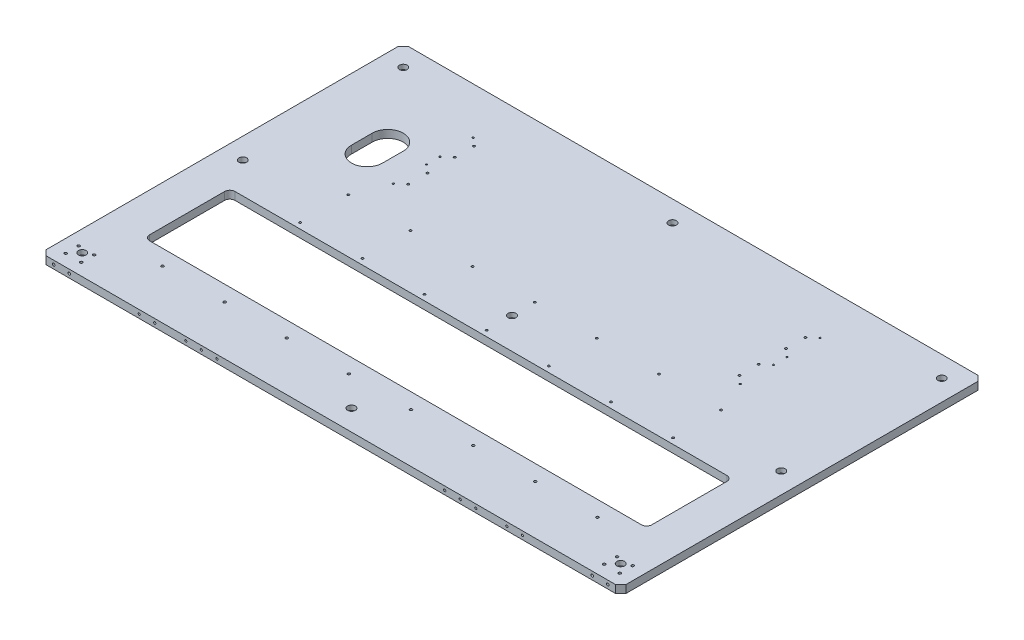
SolidWorks part; units mm, degrees
material "S45C"
ref_plane "前视基准面" through (0, 0, 0) normal (0, 0, 1) x (1, 0, 0)
ref_plane "上视基准面" through (0, 0, 0) normal (0, 1, 0) x (1, 0, 0)
ref_plane "右视基准面" through (0, 0, 0) normal (1, 0, 0) x (0, 0, -1)
sketch "草图1" plane through (0, 0, 0) normal (0, 1, 0) x (1, 0, 0)
  line L1 (-560, 350) -> (560, 350)
  line L2 (-560, 350) -> (-560, -350)
  line L3 (-560, -350) -> (560, -350)
  line L4 (560, 350) -> (560, -350)
  line L5 (-560, 350) -> (560, -350) construction
  line L6 (-560, -350) -> (560, 350) construction
  point P0 (0, 0)
  dimension "D1" = 1120
  dimension "D2" = 700
extrude "凸台-拉伸1" add sketch "草图1" along normal blind 15
chamfer "倒角1" distance 10 angle 45 4 edges at (-560, 7.5, -350) (560, 7.5, -350) (560, 7.5, 350) (-560, 7.5, 350)
sketch "草图2" plane through (0, 15, 0) normal (0, 1, 0) x (1, 0, 0)
  line L0 (560, -340) -> (560, 340) construction
  line L1 (485, -60) -> (-485, -60)
  line L2 (485, -60) -> (485, -225)
  line L3 (485, -225) -> (-485, -225)
  line L4 (-485, -60) -> (-485, -225)
  line L5 (-560, 340) -> (-560, -340) construction
  line L6 (-550, -350) -> (550, -350) construction
  dimension "D1" = 75
  dimension "D2" = 75
  dimension "D3" = 125
  dimension "D4" = 165
extrude "切除-拉伸1" cut sketch "草图2" against normal blind 20
fillet "圆角1" radius 10 4 edges at (485, 7.5, 60) (485, 7.5, 225) (-485, 7.5, 225) (-485, 7.5, 60)
hole_wizard "打孔尺寸(%根据)内六角圆柱头螺钉的类型1" positions "草图3" profile "草图4" counterbore size "M8" standard "GB"
sketch "草图3" plane through (0, 15, 0) normal (0, 1, 0) x (1, 0, 0)
  point P0 (520, -310)
  point P3 (520, 0)
  point P6 (520, 310)
  point P9 (-520, -310)
  point P12 (-520, 0)
  point P15 (-520, 310)
sketch "草图4" plane through (520, 15, 310) normal (1, 0, 0) x (0, 0, 1)
  line L0 (0, 0) -> (0, 22.4539)
  line L1 (0, 22.4539) -> (4.5, 19.75)
  line L2 (4.5, 19.75) -> (4.5, 9)
  line L3 (4.5, 9) -> (7.5, 9)
  line L4 (7.5, 9) -> (7.5, 0)
  line L5 (7.5, 0) -> (0, 0)
  line L10 (0, 22.4539) -> (-4.5, 19.75) construction
  line L11 (0, -6.35) -> (0, 107.95) construction
  dimension "孔直径" = 9
  dimension "孔深度" = 19.75
  dimension "柱形沉头孔直径" = 15
  dimension "柱形沉头孔深度" = 9
  dimension "导头角度" = 118
hole_wizard "M6 螺纹孔1" positions "草图5" profile "草图6" tap size "M6" standard "GB"
sketch "草图5" plane through (0, 15, 0) normal (0, 1, 0) x (1, 0, 0)
  point P0 (-420, -255)
  point P3 (-300, -255)
  point P6 (-180, -255)
  point P9 (-60, -255)
  point P12 (60, -255)
  point P15 (180, -255)
  point P18 (300, -255)
  point P21 (420, -255)
sketch "草图6" plane through (-420, 15, 255) normal (1, 0, 0) x (0, 0, 1)
  line L0 (0, 0) -> (0, 16.5022)
  line L1 (0, 16.5022) -> (2.5, 15)
  line L2 (2.5, 15) -> (2.5, 0)
  line L5 (2.5, 0) -> (0, 0)
  line L10 (0, 16.5022) -> (-2.5, 15) construction
  line L11 (0, -6.35) -> (0, 107.95) construction
  dimension "螺纹孔钻头直径" = 5
  dimension "螺纹孔钻头深度" = 15
  dimension "导头角度" = 118
cosmetic thread "孔螺蚊线31" parameters "D1"=12, "D2"=6
cosmetic thread "孔螺蚊线32" parameters "D1"=12, "D2"=6
cosmetic thread "孔螺蚊线33" parameters "D1"=12, "D2"=6
cosmetic thread "孔螺蚊线34" parameters "D1"=12, "D2"=6
cosmetic thread "孔螺蚊线35" parameters "D1"=12, "D2"=6
cosmetic thread "孔螺蚊线36" parameters "D1"=12, "D2"=6
cosmetic thread "孔螺蚊线37" parameters "D1"=12, "D2"=6
cosmetic thread "孔螺蚊线38" parameters "D1"=12, "D2"=6
hole_wizard "M5 螺纹孔1" positions "草图7" profile "草图8" tap size "M5" standard "GB"
sketch "草图7" plane through (0, 15, 0) normal (0, 1, 0) x (1, 0, 0)
  point P0 (360, -49)
  point P3 (360, 44)
  point P6 (240, -49)
  point P9 (240, 44)
  point P12 (120, -49)
  point P15 (120, 44)
  point P18 (0, -49)
  point P21 (0, 44)
  point P24 (-120, -49)
  point P27 (-120, 44)
  point P30 (-240, -49)
  point P33 (-240, 44)
  point P36 (-360, -49)
  point P39 (-360, 44)
sketch "草图8" plane through (360, 15, 49) normal (1, 0, 0) x (0, 0, 1)
  line L0 (0, 0) -> (0, 21.2618)
  line L1 (0, 21.2618) -> (2.1, 20)
  line L2 (2.1, 20) -> (2.1, 0)
  line L5 (2.1, 0) -> (0, 0)
  line L10 (0, 21.2618) -> (-2.1, 20) construction
  line L11 (0, -6.35) -> (0, 107.95) construction
  dimension "螺纹孔钻头直径" = 4.2
  dimension "螺纹孔钻头深度" = 20
  dimension "导头角度" = 118
cosmetic thread "孔螺蚊线9" parameters "D1"=10, "D2"=5
cosmetic thread "孔螺蚊线10" parameters "D1"=10, "D2"=5
cosmetic thread "孔螺蚊线11" parameters "D1"=10, "D2"=5
cosmetic thread "孔螺蚊线12" parameters "D1"=10, "D2"=5
cosmetic thread "孔螺蚊线13" parameters "D1"=10, "D2"=5
cosmetic thread "孔螺蚊线14" parameters "D1"=10, "D2"=5
cosmetic thread "孔螺蚊线15" parameters "D1"=10, "D2"=5
cosmetic thread "孔螺蚊线16" parameters "D1"=10, "D2"=5
cosmetic thread "孔螺蚊线17" parameters "D1"=10, "D2"=5
cosmetic thread "孔螺蚊线18" parameters "D1"=10, "D2"=5
cosmetic thread "孔螺蚊线19" parameters "D1"=10, "D2"=5
cosmetic thread "孔螺蚊线20" parameters "D1"=10, "D2"=5
cosmetic thread "孔螺蚊线21" parameters "D1"=10, "D2"=5
cosmetic thread "孔螺蚊线22" parameters "D1"=10, "D2"=5
sketch "草图9" plane through (0, 15, 0) normal (0, 1, 0) x (1, 0, 0)
  line L0 (-410, 130) -> (-410, 170) construction
  line L1 (-440, 130) -> (-440, 170)
  line L2 (-380, 130) -> (-380, 170)
  line L3 (550, 350) -> (-550, 350) construction
  line L4 (-560, 340) -> (-560, -340) construction
  arc A0 (-440, 130) -> (-380, 130) centre (-410, 130) ccw
  arc A1 (-380, 170) -> (-440, 170) centre (-410, 170) ccw
  point P2 (-410, 150)
  dimension "D1" = 180
  dimension "D3" = 150
  dimension "D4" = 30
  dimension "D2" = 40
extrude "切除-拉伸2" cut sketch "草图9" against normal blind 20
hole_wizard "M5 螺纹孔2" positions "草图10" profile "草图11" tap size "M5" standard "GB"
sketch "草图10" plane through (0, 0, 350) normal (0, 0, 1) x (1, 0, 0)
  line L1 (-550, 15) -> (550, 15) construction
  line L2 (560, 15) -> (560, 0) construction
  point P0 (-280, 7.5)
  point P3 (-250, 7.5)
  point P6 (-220, 7.5)
  point P10 (280, 7.5)
  point P12 (250, 7.5)
  point P14 (220, 7.5)
  dimension "D1" = 30
  dimension "D2" = 30
  dimension "D3" = 7.5
  dimension "D4" = 280
sketch "草图11" plane through (-280, 7.5, 350) normal (1, 0, 0) x (0, -1, 0)
  line L0 (0, 0) -> (0, 21.2618)
  line L1 (0, 21.2618) -> (2.1, 20)
  line L2 (2.1, 20) -> (2.1, 0)
  line L5 (2.1, 0) -> (0, 0)
  line L10 (0, 21.2618) -> (-2.1, 20) construction
  line L11 (0, -6.35) -> (0, 107.95) construction
  dimension "螺纹孔钻头直径" = 4.2
  dimension "螺纹孔钻头深度" = 20
  dimension "导头角度" = 118
cosmetic thread "孔螺蚊线39" parameters "D1"=10, "D2"=5
cosmetic thread "孔螺蚊线40" parameters "D1"=10, "D2"=5
cosmetic thread "孔螺蚊线41" parameters "D1"=10, "D2"=5
cosmetic thread "孔螺蚊线58" parameters "D1"=10, "D2"=5
cosmetic thread "孔螺蚊线59" parameters "D1"=10, "D2"=5
cosmetic thread "孔螺蚊线60" parameters "D1"=10, "D2"=5
hole_wizard "M4 螺纹孔1" positions "草图12" profile "草图13" tap size "M4" standard "GB"
sketch "草图12" plane through (0, 15, 0) normal (0, 1, 0) x (1, 0, 0)
  point P0 (335, 106)
  point P3 (335, 170)
  point P6 (-335, 106)
  point P9 (-335, 170)
  point P12 (-335, 196)
  point P15 (-335, 260)
  point P18 (335, 196)
  point P21 (335, 260)
sketch "草图13" plane through (335, 15, -106) normal (1, 0, 0) x (0, 0, 1)
  line L0 (0, 0) -> (0, 20.9914)
  line L1 (0, 20.9914) -> (1.65, 20)
  line L2 (1.65, 20) -> (1.65, 0)
  line L5 (1.65, 0) -> (0, 0)
  line L10 (0, 20.9914) -> (-1.65, 20) construction
  line L11 (0, -6.35) -> (0, 107.95) construction
  dimension "螺纹孔钻头直径" = 3.3
  dimension "螺纹孔钻头深度" = 20
  dimension "导头角度" = 118
cosmetic thread "孔螺蚊线42" parameters "D1"=8, "D2"=4
cosmetic thread "孔螺蚊线43" parameters "D1"=8, "D2"=4
cosmetic thread "孔螺蚊线44" parameters "D1"=8, "D2"=4
cosmetic thread "孔螺蚊线45" parameters "D1"=8, "D2"=4
cosmetic thread "孔螺蚊线46" parameters "D1"=8, "D2"=4
cosmetic thread "孔螺蚊线47" parameters "D1"=8, "D2"=4
cosmetic thread "孔螺蚊线48" parameters "D1"=8, "D2"=4
cosmetic thread "孔螺蚊线49" parameters "D1"=8, "D2"=4
hole_wizard "M5 螺纹孔3" positions "草图14" profile "草图15" tap size "M5" standard "GB"
sketch "草图14" plane through (0, 15, 0) normal (0, 1, 0) x (1, 0, 0)
  point P0 (320, 119.5)
  point P3 (320, 156.5)
  point P6 (320, 209.5)
  point P9 (320, 246.5)
  point P12 (-320, 119.5)
  point P15 (-320, 156.5)
  point P18 (-320, 209.5)
  point P21 (-320, 246.5)
sketch "草图15" plane through (320, 15, -119.5) normal (1, 0, 0) x (0, 0, 1)
  line L0 (0, 0) -> (0, 21.2618)
  line L1 (0, 21.2618) -> (2.1, 20)
  line L2 (2.1, 20) -> (2.1, 0)
  line L5 (2.1, 0) -> (0, 0)
  line L10 (0, 21.2618) -> (-2.1, 20) construction
  line L11 (0, -6.35) -> (0, 107.95) construction
  dimension "螺纹孔钻头直径" = 4.2
  dimension "螺纹孔钻头深度" = 20
  dimension "导头角度" = 118
cosmetic thread "孔螺蚊线50" parameters "D1"=10, "D2"=5
cosmetic thread "孔螺蚊线51" parameters "D1"=10, "D2"=5
cosmetic thread "孔螺蚊线52" parameters "D1"=10, "D2"=5
cosmetic thread "孔螺蚊线53" parameters "D1"=10, "D2"=5
cosmetic thread "孔螺蚊线54" parameters "D1"=10, "D2"=5
cosmetic thread "孔螺蚊线55" parameters "D1"=10, "D2"=5
cosmetic thread "孔螺蚊线56" parameters "D1"=10, "D2"=5
cosmetic thread "孔螺蚊线57" parameters "D1"=10, "D2"=5
hole_wizard "M5 螺纹孔4" positions "草图16" profile "草图17" tap size "M5" standard "GB"
sketch "草图16" plane through (0, 0, 350) normal (0, 0, 1) x (1, 0, 0)
  line L0 (-550, 15) -> (550, 15) construction
  line L1 (-560, 0) -> (-560, 15) construction
  line L2 (560, 15) -> (560, 0) construction
  point P0 (-370, 7.5)
  point P2 (-340, 7.5)
  point P4 (370, 7.5)
  point P6 (340, 7.5)
  dimension "D1" = 7.5
  dimension "D2" = 30
  dimension "D3" = 190
  dimension "D4" = 7.5
  dimension "D5" = 30
  dimension "D6" = 190
sketch "草图17" plane through (-370, 7.5, 350) normal (1, 0, 0) x (0, -1, 0)
  line L0 (0, 0) -> (0, 13.6618)
  line L1 (0, 13.6618) -> (2.1, 12.4)
  line L2 (2.1, 12.4) -> (2.1, 0)
  line L5 (2.1, 0) -> (0, 0)
  line L10 (0, 13.6618) -> (-2.1, 12.4) construction
  line L11 (0, -6.35) -> (0, 107.95) construction
  dimension "螺纹孔钻头直径" = 4.2
  dimension "螺纹孔钻头深度" = 12.4
  dimension "导头角度" = 118
cosmetic thread "孔螺蚊线61" parameters "D1"=10, "D2"=5
cosmetic thread "孔螺蚊线62" parameters "D1"=10, "D2"=5
cosmetic thread "孔螺蚊线63" parameters "D1"=10, "D2"=5
cosmetic thread "孔螺蚊线64" parameters "D1"=10, "D2"=5
hole_wizard "打孔尺寸(%根据)内六角圆柱头螺钉的类型2" positions "草图18" profile "草图19" counterbore size "M8" standard "GB"
sketch "草图18" plane through (0, 15, 0) normal (0, 1, 0) x (1, 0, 0)
  point P0 (0, 310)
  point P3 (0, 0)
  point P6 (0, -310)
sketch "草图19" plane through (0, 15, -310) normal (1, 0, 0) x (0, 0, 1)
  line L0 (0, 0) -> (0, 22.4539)
  line L1 (0, 22.4539) -> (4.5, 19.75)
  line L2 (4.5, 19.75) -> (4.5, 9)
  line L3 (4.5, 9) -> (7.5, 9)
  line L4 (7.5, 9) -> (7.5, 0)
  line L5 (7.5, 0) -> (0, 0)
  line L10 (0, 22.4539) -> (-4.5, 19.75) construction
  line L11 (0, -6.35) -> (0, 107.95) construction
  dimension "孔直径" = 9
  dimension "孔深度" = 19.75
  dimension "柱形沉头孔直径" = 15
  dimension "柱形沉头孔深度" = 9
  dimension "导头角度" = 118
hole_wizard "M6 螺纹孔2" positions "草图20" profile "草图21" tap size "M6" standard "GB"
sketch "草图20" plane through (0, 0, 350) normal (0, 0, 1) x (1, 0, 0)
  point P0 (-535, 7.5)
  point P3 (-505, 7.5)
  point P6 (505, 7.5)
  point P9 (535, 7.5)
cosmetic thread "孔螺蚊线65"
cosmetic thread "孔螺蚊线66"
cosmetic thread "孔螺蚊线67"
cosmetic thread "孔螺蚊线68"
sketch "草图21" plane through (-535, 7.5, 350) normal (1, 0, 0) x (0, -1, 0)
  line L0 (0, 0) -> (0, 16.5022)
  line L1 (0, 16.5022) -> (2.5, 15)
  line L2 (2.5, 15) -> (2.5, 0)
  line L5 (2.5, 0) -> (0, 0)
  line L10 (0, 16.5022) -> (-2.5, 15) construction
  line L11 (0, -6.35) -> (0, 107.95) construction
  dimension "螺纹孔钻头直径" = 5
  dimension "螺纹孔钻头深度" = 15
  dimension "导头角度" = 118
hole_wizard "M6 螺纹孔3" positions "草图22" profile "草图23" tap size "M6" standard "GB"
sketch "草图22" plane through (0, 15, 0) normal (0, 1, 0) x (1, 0, 0)
  point P0 (535, -327)
  point P3 (505, -327)
  point P6 (535, -302)
  point P9 (505, -302)
  point P12 (-505, -327)
  point P15 (-535, -327)
  point P18 (-505, -302)
  point P21 (-535, -302)
sketch "草图23" plane through (535, 15, 327) normal (1, 0, 0) x (0, 0, 1)
  line L0 (0, 0) -> (0, 16.5022)
  line L1 (0, 16.5022) -> (2.5, 15)
  line L2 (2.5, 15) -> (2.5, 0)
  line L5 (2.5, 0) -> (0, 0)
  line L10 (0, 16.5022) -> (-2.5, 15) construction
  line L11 (0, -6.35) -> (0, 107.95) construction
  dimension "螺纹孔钻头直径" = 5
  dimension "螺纹孔钻头深度" = 15
  dimension "导头角度" = 118
cosmetic thread "孔螺蚊线69"
cosmetic thread "孔螺蚊线70"
cosmetic thread "孔螺蚊线71"
cosmetic thread "孔螺蚊线72"
cosmetic thread "孔螺蚊线73"
cosmetic thread "孔螺蚊线74"
cosmetic thread "孔螺蚊线75"
cosmetic thread "孔螺蚊线76"
